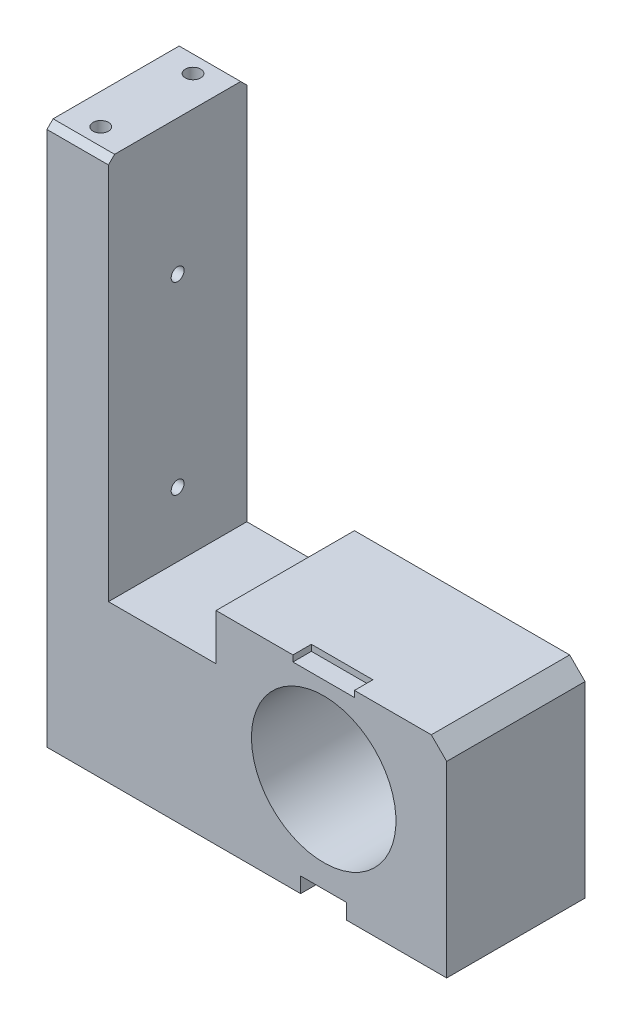
from build123d import *

# Parameters (mm, degrees)
SKETCH1_R             = 23.5
BOSS_EXTRUDE1_DEPTH   = 45
M6_TAPPED_HOLE1_D     = 5
M6_TAPPED_HOLE1_DEPTH = 15
M6_TAPPED_HOLE1_TIP   = 1.502151548
M5_TAPPED_HOLE1_D     = 4.2
M6_TAPPED_HOLE2_D     = 5
M6_TAPPED_HOLE2_DEPTH = 15
M6_TAPPED_HOLE2_TIP   = 1.502151548
M4_TAPPED_HOLE1_D     = 3.3
M4_TAPPED_HOLE1_DEPTH = 10.1
M4_TAPPED_HOLE1_TIP   = 0.991420021
CHAMFER1_SIZE         = 5
CHAMFER2_SIZE         = 2
SKETCH18_W            = 35
SKETCH18_H            = 15
CUT_EXTRUDE1_DEPTH    = 173.409396496
SKETCH19_W            = 20
SKETCH19_H            = 6
CUT_EXTRUDE2_DEPTH    = 2


with BuildPart() as part:
    # Sketch1 → Boss-Extrude1 (new body)
    with BuildSketch(Plane.XY):
        Polygon((-90, 140), (-90, -36), (-7.5, -36), (-7.5, -31), (7.5, -31), (7.5, -36), (40, -36), (40, 30), (-70, 30), (-70, 140), align=None)
        with Locations(Location((0, 0, 0), (0, 0, 180))):
            Circle(SKETCH1_R, mode=Mode.SUBTRACT)
    extrude(amount=BOSS_EXTRUDE1_DEPTH)

    # M6 Tapped Hole1
    with Locations(Plane.XZ.offset(36)):
        with Locations((-75, 10), (25, 10), (-75, 35), (25, 35)):
            Hole(M6_TAPPED_HOLE1_D / 2, depth=M6_TAPPED_HOLE1_DEPTH)
            with Locations((0, 0, -(M6_TAPPED_HOLE1_DEPTH + M6_TAPPED_HOLE1_TIP / 2))):  # 118° drill point
                Cone(0, M6_TAPPED_HOLE1_D / 2, M6_TAPPED_HOLE1_TIP, mode=Mode.SUBTRACT)

    # M5 Tapped Hole1 (through all)
    with Locations(Plane(origin=(-70, 0, 0), x_dir=(0, 0, -1), z_dir=(1, 0, 0))):
        with Locations((-22.5, 96), (-22.5, 36)):
            Hole(M5_TAPPED_HOLE1_D / 2)

    # M6 Tapped Hole2
    with Locations(Plane(origin=(0, 140, 0), x_dir=(-1, 0, 0), z_dir=(0, 1, 0))):
        with Locations((80, 7.5), (80, 37.5)):
            Hole(M6_TAPPED_HOLE2_D / 2, depth=M6_TAPPED_HOLE2_DEPTH)
            with Locations((0, 0, -(M6_TAPPED_HOLE2_DEPTH + M6_TAPPED_HOLE2_TIP / 2))):  # 118° drill point
                Cone(0, M6_TAPPED_HOLE2_D / 2, M6_TAPPED_HOLE2_TIP, mode=Mode.SUBTRACT)

    # M4 Tapped Hole1
    with Locations(Plane(origin=(0, 0, 0), x_dir=(-1, 0, 0), z_dir=(0, 0, -1))):
        with Locations((-19.445436483, 19.445436483), (19.445436483, -19.445436483), (-19.445436483, -19.445436483), (19.445436483, 19.445436483)):
            Hole(M4_TAPPED_HOLE1_D / 2, depth=M4_TAPPED_HOLE1_DEPTH)
            with Locations((0, 0, -(M4_TAPPED_HOLE1_DEPTH + M4_TAPPED_HOLE1_TIP / 2))):  # 118° drill point
                Cone(0, M4_TAPPED_HOLE1_D / 2, M4_TAPPED_HOLE1_TIP, mode=Mode.SUBTRACT)

    # Chamfer1
    chamfer1_edges = [part.edges().sort_by_distance(p)[0] for p in [
        (40, 30, 22.5),
    ]]
    chamfer(chamfer1_edges, length=CHAMFER1_SIZE)

    # Chamfer2
    chamfer2_edges = [part.edges().sort_by_distance(p)[0] for p in [
        (-80, 140, 45),
        (-80, 140, 0),
    ]]
    chamfer(chamfer2_edges, length=CHAMFER2_SIZE)

    # Sketch18 → Cut-Extrude1 (cut, through all)
    with BuildSketch(Plane(origin=(0, 0, 0), x_dir=(-1, 0, 0), z_dir=(0, 0, -1))):
        with Locations((52.5, 22.5)):
            Rectangle(SKETCH18_W, SKETCH18_H)
    extrude(amount=-CUT_EXTRUDE1_DEPTH, mode=Mode.SUBTRACT)

    # Sketch19 → Cut-Extrude2 (cut)
    with BuildSketch(Plane(origin=(0, 30, 0), x_dir=(1, 0, 0), z_dir=(0, 1, 0))):
        with Locations((0, -42)):
            Rectangle(SKETCH19_W, SKETCH19_H)
    extrude(amount=-CUT_EXTRUDE2_DEPTH, mode=Mode.SUBTRACT)


solid = part.part
